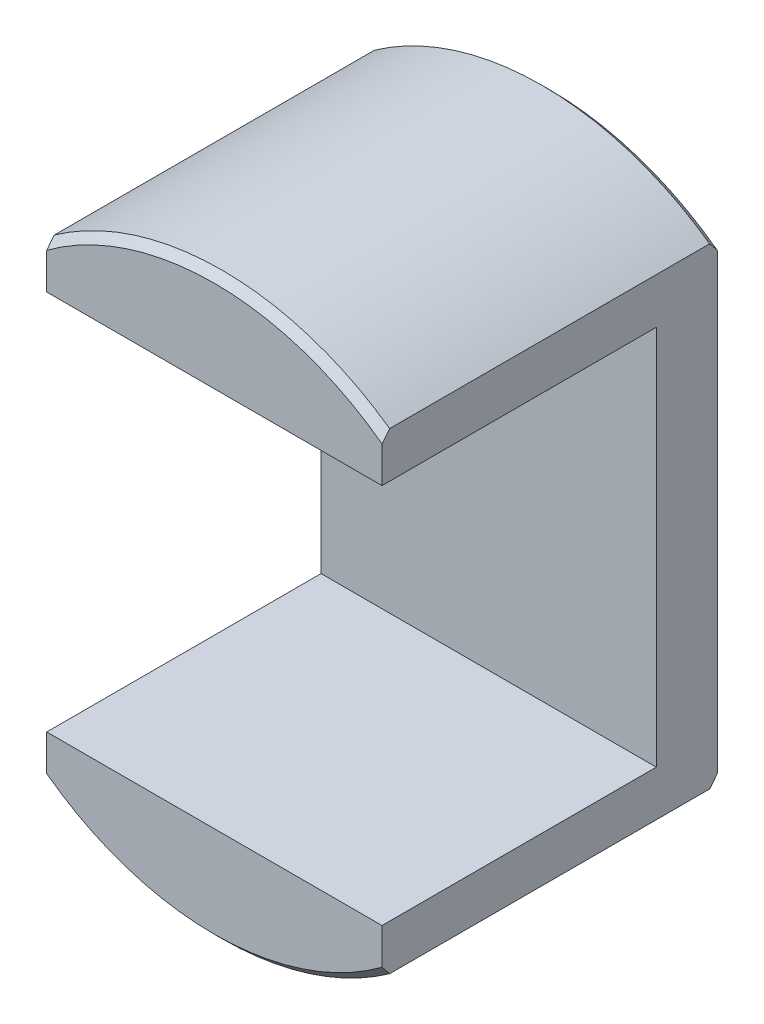
SolidWorks part; units mm, degrees
ref_plane "Front Plane" through (0, 0, 0) normal (0, 0, 1) x (1, 0, 0)
ref_plane "Top Plane" through (0, 0, 0) normal (0, 1, 0) x (1, 0, 0)
ref_plane "Right Plane" through (0, 0, 0) normal (1, 0, 0) x (0, 0, -1)
other "Configuration Table"
sketch "Sketch1" plane through (0, 0, 0) normal (0, 0, 1) x (1, 0, 0)
  line L0 (-11, 4.3159) -> (11, 4.3159) construction
  line L2 (11, -15.4919) -> (11, 15.4919)
  line L4 (-11, -15.4919) -> (-11, 15.4919)
  line L5 (6.1997, -17.96) -> (-6.1997, 17.96) construction
  line L6 (6.1997, 17.96) -> (-6.1997, -17.96) construction
  arc A0 (-11, -15.4919) -> (11, -15.4919) centre (0, 0) ccw
  arc A1 (11, 15.4919) -> (-11, 15.4919) centre (0, 0) ccw
  point P6 (0, 4.3159)
  dimension "D1" = 38
  dimension "D2" = 22
extrude "Boss-Extrude1" add sketch "Sketch1" along normal blind 22
sketch "Sketch2" plane through (0, 0, 22) normal (0, 0, 1) x (1, 0, 0)
  line L0 (-11, 15.4919) -> (-11, -15.4919) construction
  line L1 (11, -12.5) -> (-11, -12.5)
  line L2 (11, -12.5) -> (11, 12.5)
  line L3 (11, 12.5) -> (-11, 12.5)
  line L4 (-11, -12.5) -> (-11, 12.5)
  line L5 (11, -12.5) -> (-11, 12.5) construction
  line L6 (11, 12.5) -> (-11, -12.5) construction
  point P0 (0, 0)
  dimension "D1" = 25
extrude "Cut-Extrude1" cut sketch "Sketch2" against normal blind 18
chamfer "Chamfer1" distance 0.5 angle 45 4 edges at (0, -19, 0) (0, -19, 22) (0, 19, 0) (0, 19, 22)
